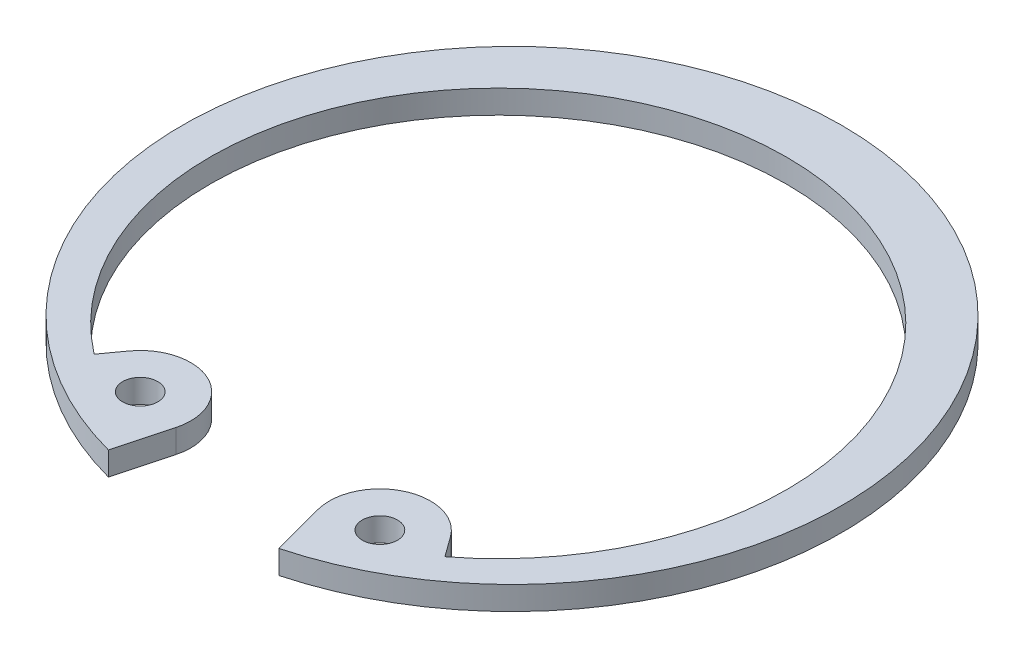
SolidWorks part; units mm, degrees
ref_plane "Front Plane" through (0, 0, 0) normal (0, 0, 1) x (1, 0, 0)
ref_plane "Top Plane" through (0, 0, 0) normal (0, 1, 0) x (1, 0, 0)
ref_plane "Right Plane" through (0, 0, 0) normal (1, 0, 0) x (0, 0, -1)
sketch "Sketch1" plane through (0, 0, 0) normal (0, 0, 1) x (1, 0, 0)
  line L1 (0, 0) -> (56.2, 0)
  line L2 (0, 0) -> (0, 2)
  line L3 (0, 2) -> (56.2, 2)
  line L4 (56.2, 0) -> (56.2, 2)
  line L5 (0, 0) -> (4.7, 0)
  line L6 (0, 0) -> (0, 3)
  line L7 (0, 3) -> (4.7, 3)
  line L8 (4.7, 0) -> (4.7, 3)
  dimension "D3" = 56.2
  dimension "T" = 2
  dimension "C" = 4.7
  dimension "D0" = 3
sketch "Sketch2" plane through (0, 0, 0) normal (0, 1, 0) x (1, 0, 0)
  line L0 (0, 28.1) -> (0, 23.4) construction
  line L1 (-14.9539, -20.6765) -> (-13.7109, -18.9578)
  line L2 (-6.0554, -22.5991) -> (-7.2728, -27.1425)
  line L3 (0, 1.6194) -> (0, -3.957) construction
  line L4 (6.0554, -22.5991) -> (7.2728, -27.1425)
  line L5 (0, 0) -> (-10.2186, -21.4836) construction
  line L6 (14.9539, -20.6765) -> (13.7109, -18.9578)
  arc A0 (7.2728, -27.1425) -> (-7.2728, -27.1425) centre (0, 0) ccw
  arc A2 (-6.0554, -22.5991) -> (-13.7109, -18.9578) centre (-10.2186, -21.4836) ccw
  circle A3 centre (-10.2186, -21.4836) radius 1.5
  circle A4 centre (10.2186, -21.4836) radius 1.5
  arc A5 (6.0554, -22.5991) -> (13.7109, -18.9578) centre (10.2186, -21.4836) cw
  arc A7 (14.9539, -20.6765) -> (-14.9539, -20.6765) centre (0, -1.175) ccw
  dimension "D1" = 56.2
  dimension "D3" = 49.15
  dimension "D5" = 3
  dimension "D6" = 8.62
  dimension "D2" = 4.7
  dimension "D4" = 15
  dimension "D7" = 23.79
extrude "Boss-Extrude1" add sketch "Sketch2" along normal blind 2
